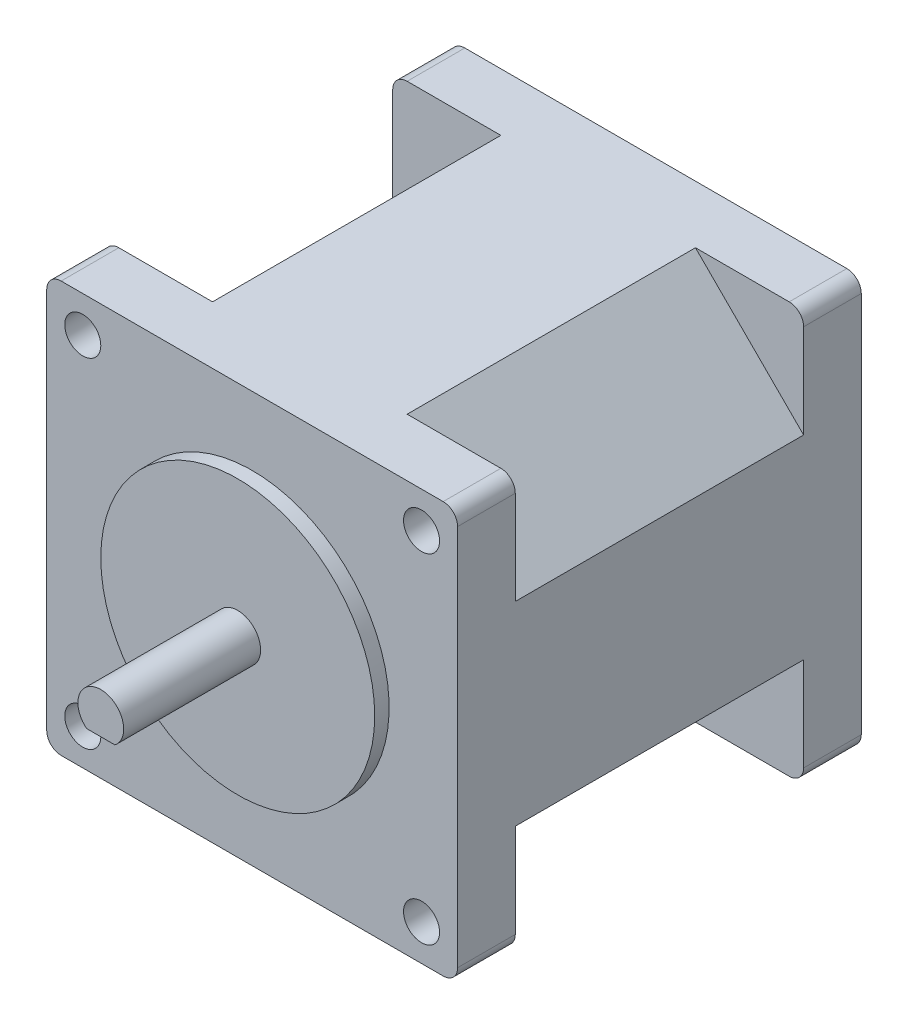
from build123d import *

# Parameters (mm, degrees)
SKETCH_1_W               = 57
SKETCH_1_H               = 57
EXTRUDE_1_DEPTH          = 56
SKETCH_2_R               = 19
EXTRUDE_2_DEPTH          = 2
SKETCH_3_R               = 3.175
EXTRUDE_3_DEPTH          = 19
CUT_EXTRUDE_1_DEPTH      = 20
SKETCH_5_R               = 2.5
CUT_EXTRUDE_2_DEPTH      = 8
PATTERN_CIRCULAR_1_COUNT = 4
FILLET_1_R               = 2
SKETCH_6_W               = 11.376711671
SKETCH_6_H               = 3.467188319
CUT_EXTRUDE_3_DEPTH      = 15


with BuildPart() as part:
    # 草图1 → 凸台-拉伸1 (new body)
    with BuildSketch(Plane.XY):
        Rectangle(SKETCH_1_W, SKETCH_1_H)
    extrude(amount=EXTRUDE_1_DEPTH)

    # 草图2 → 凸台-拉伸2 (add)
    with BuildSketch(Plane.XY.offset(56)):
        with Locations(Location((0, 0, 0), (0, 0, 180))):
            Circle(SKETCH_2_R)
    extrude(amount=EXTRUDE_2_DEPTH)

    # 草图3 → 凸台-拉伸3 (add)
    with BuildSketch(Plane.XY.offset(58)):
        Circle(SKETCH_3_R)
    extrude(amount=EXTRUDE_3_DEPTH)

    # 草图4 → 切除-拉伸1 (cut, symmetric)
    with BuildSketch(Plane.XY.offset(28)):
        Polygon((13.5, 28.5), (28.5, 13.5), (28.5, 28.5), align=None)
    cut_extrude_1 = extrude(amount=CUT_EXTRUDE_1_DEPTH, both=True, mode=Mode.SUBTRACT)

    # 草图5 → 切除-拉伸2 (cut)
    with BuildSketch(Plane.XY.offset(56)):
        with Locations((23.5, 23.5)):
            Circle(SKETCH_5_R)
    cut_extrude_2 = extrude(amount=-CUT_EXTRUDE_2_DEPTH, mode=Mode.SUBTRACT)

    # 阵列(圆周)1: 切除-拉伸1, 切除-拉伸2 ×4 about axis
    pattern_circular_1_axis = Axis((0, 0, 0), (0, 0, 1))
    add([cut_extrude_1.rotate(pattern_circular_1_axis, i * 360 / PATTERN_CIRCULAR_1_COUNT) for i in range(1, PATTERN_CIRCULAR_1_COUNT)], mode=Mode.SUBTRACT)
    add([cut_extrude_2.rotate(pattern_circular_1_axis, i * 360 / PATTERN_CIRCULAR_1_COUNT) for i in range(1, PATTERN_CIRCULAR_1_COUNT)], mode=Mode.SUBTRACT)

    # 圆角1
    fillet_1_edges = [part.edges().sort_by_distance(p)[0] for p in [
        (28.5, 28.5, 4),
        (28.5, -28.5, 4),
        (-28.5, -28.5, 4),
        (-28.5, 28.5, 4),
        (28.5, -28.5, 52),
        (-28.5, -28.5, 52),
        (-28.5, 28.5, 52),
        (28.5, 28.5, 52),
    ]]
    fillet(fillet_1_edges, radius=FILLET_1_R)

    # 草图6 → 切除-拉伸3 (cut)
    with BuildSketch(Plane.XY.offset(77)):
        with Locations((0.056540367, -4.23359416)):
            Rectangle(SKETCH_6_W, SKETCH_6_H)
    extrude(amount=-CUT_EXTRUDE_3_DEPTH, mode=Mode.SUBTRACT)


solid = part.part
